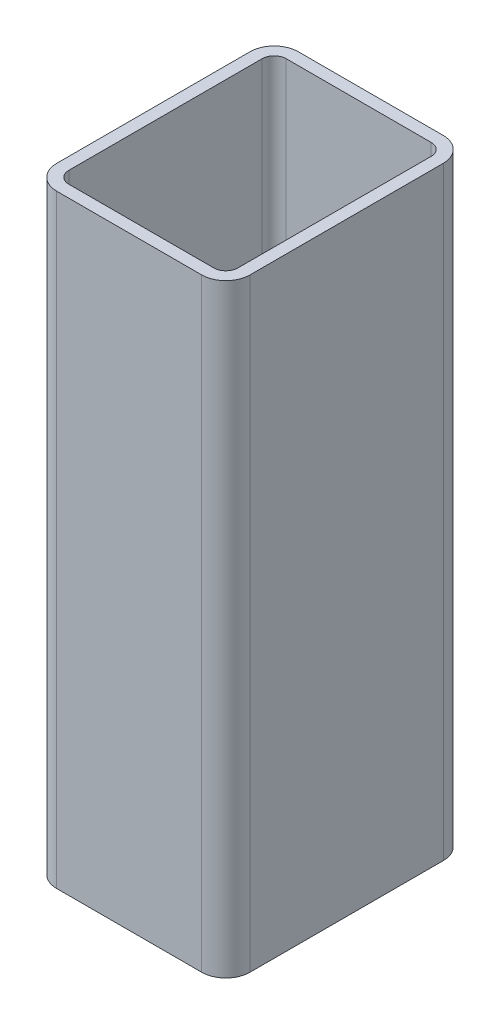
SolidWorks part; units mm, degrees
material "Q235B"
ref_plane "Front Plane" through (0, 0, 0) normal (0, 0, 1) x (1, 0, 0)
ref_plane "Top Plane" through (0, 0, 0) normal (0, 1, 0) x (1, 0, 0)
ref_plane "Right Plane" through (0, 0, 0) normal (1, 0, 0) x (0, 0, -1)
sketch "Sketch1" plane through (0, 0, 0) normal (0, 0, 1) x (1, 0, 0)
  line L0 (0, 0) -> (0, 250)
  dimension "D1" = 250
other "Gb／t 6728—2002 rectangular hollow section 100X80X5(1)"
ref_plane "Plane1" through (0, 0, 0) normal (0, 1, 0) x (-1, 0, 0)
sketch "Sketch12" plane through (0, 0, 0) normal (0, 1, 0) x (-1, 0, 0)
  line L0 (-30, -45) -> (30, -45)
  line L1 (-35, -40) -> (-35, 40)
  line L2 (30, 45) -> (-30, 45)
  line L3 (35, 40) -> (35, -40)
  line L4 (-30, -50) -> (30, -50)
  line L5 (-40, -40) -> (-40, 40)
  line L6 (30, 50) -> (-30, 50)
  line L7 (40, 40) -> (40, -40)
  arc A0 (40, 40) -> (30, 50) centre (30, 40) ccw
  arc A1 (30, -50) -> (40, -40) centre (30, -40) ccw
  arc A2 (-40, -40) -> (-30, -50) centre (-30, -40) ccw
  arc A3 (-30, 50) -> (-40, 40) centre (-30, 40) ccw
  arc A4 (-30, 45) -> (-35, 40) centre (-30, 40) ccw
  arc A5 (35, 40) -> (30, 45) centre (30, 40) ccw
  arc A6 (30, -45) -> (35, -40) centre (30, -40) ccw
  arc A7 (-35, -40) -> (-30, -45) centre (-30, -40) ccw
  point P0 (0, 50)
  point P1 (40, 0)
  point P2 (0, -50)
  point P3 (-40, 0)
  point P4 (-40, 50)
  point P5 (40, 50)
  point P6 (40, -50)
  point P7 (-40, -50)
  point P8 (0, 0)
  point P33 (0, 0)
  dimension "D1" = 10
  dimension "Thickness" = 5
  dimension "V_leg" = 100
  dimension "H_leg" = 80
